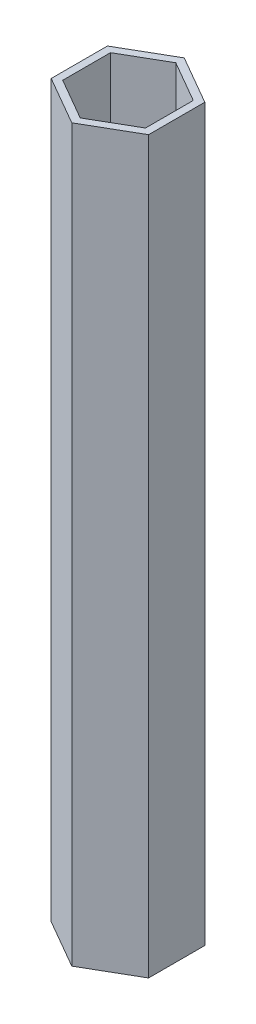
SolidWorks part; units mm, degrees
material "45"
ref_plane "Front Plane" through (0, 0, 0) normal (0, 0, 1) x (1, 0, 0)
ref_plane "Top Plane" through (0, 0, 0) normal (0, 1, 0) x (1, 0, 0)
ref_plane "Right Plane" through (0, 0, 0) normal (1, 0, 0) x (0, 0, -1)
sketch "Sketch1" plane through (0, 0, 0) normal (0, 1, 0) x (1, 0, 0)
  line L0 (-17, 9.815) -> (-17, -9.815)
  line L1 (0, 23.094) -> (-20, 11.547)
  line L2 (-20, 11.547) -> (-20, -11.547)
  line L3 (-20, -11.547) -> (0, -23.094)
  line L4 (0, -23.094) -> (20, -11.547)
  line L5 (20, -11.547) -> (20, 11.547)
  line L6 (20, 11.547) -> (0, 23.094)
  line L7 (-17, -9.815) -> (0, -19.6299)
  line L8 (0, -19.6299) -> (17, -9.815)
  line L9 (17, -9.815) -> (17, 9.815)
  line L10 (17, 9.815) -> (0, 19.6299)
  line L11 (0, 19.6299) -> (-17, 9.815)
  circle A0 centre (0, 0) radius 20 construction
  dimension "D1" = 40
  dimension "D2" = 3
extrude "Boss-Extrude1" add sketch "Sketch1" along normal blind 300
